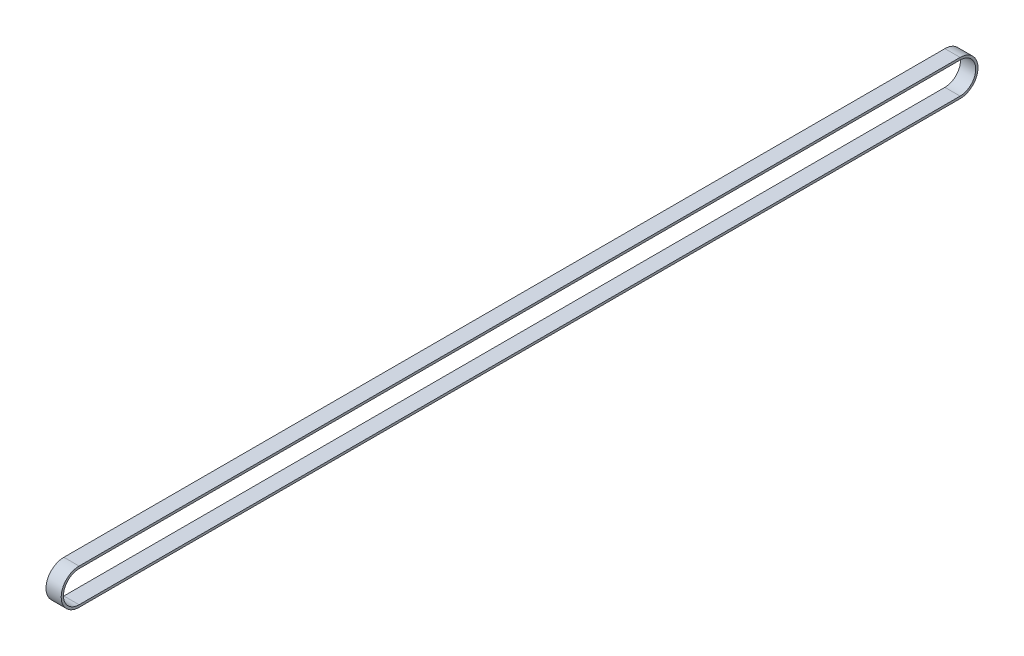
from build123d import *

# Parameters (mm, degrees)
EXTRUDE_1_DEPTH = 15


with BuildPart() as part:
    # 草图2 → 拉伸-薄壁1 (new, symmetric)
    with BuildSketch(Plane(origin=(0, 0, 0), x_dir=(0, 0, -1), z_dir=(1, 0, 0))):
        with BuildLine():
            Line((-1740, -35.35), (0, -35.35))
            ThreePointArc((0, -35.35), (35.35, 0), (0, 35.35))
            Line((0, 35.35), (-1740, 35.35))
            ThreePointArc((-1740, 35.35), (-1775.35, 0), (-1740, -35.35))
        make_face()
        with BuildLine():
            Line((-1740, -30.85), (0, -30.85))
            ThreePointArc((0, -30.85), (30.85, 0), (0, 30.85))
            Line((0, 30.85), (-1740, 30.85))
            ThreePointArc((-1740, 30.85), (-1770.85, 0), (-1740, -30.85))
        make_face(mode=Mode.SUBTRACT)
    extrude(amount=EXTRUDE_1_DEPTH, both=True)


solid = part.part
